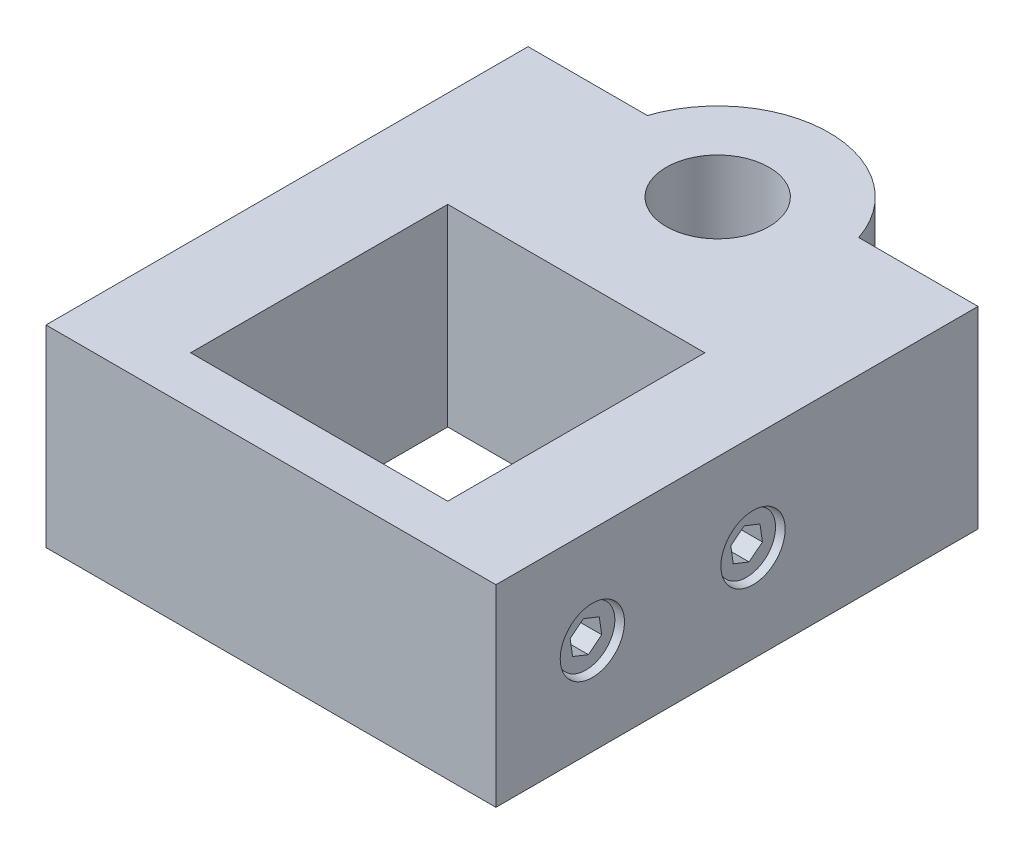
SolidWorks part; units mm, degrees
ref_plane "Front Plane" through (0, 0, 0) normal (0, 0, 1) x (1, 0, 0)
ref_plane "Top Plane" through (0, 0, 0) normal (0, 1, 0) x (1, 0, 0)
ref_plane "Right Plane" through (0, 0, 0) normal (1, 0, 0) x (0, 0, -1)
other "Configuration Table"
sketch "Sketch1" plane through (0, 0, 0) normal (0, 1, 0) x (1, 0, 0)
  line L1 (-35, 27.5) -> (35, 27.5)
  line L2 (-35, 27.5) -> (-35, -27.5)
  line L3 (-35, -27.5) -> (35, -27.5)
  line L4 (35, 27.5) -> (35, -27.5)
  line L5 (-35, 27.5) -> (35, -27.5) construction
  line L6 (-35, -27.5) -> (35, 27.5) construction
  line L7 (-20, 20) -> (20, 20)
  line L8 (-20, 20) -> (-20, -20)
  line L9 (-20, -20) -> (20, -20)
  line L10 (20, 20) -> (20, -20)
  line L11 (-20, 20) -> (20, -20) construction
  line L12 (-20, -20) -> (20, 20) construction
  point P0 (0, 0)
  point P6 (0, 0)
  dimension "D1" = 40
  dimension "D2" = 55
  dimension "D3" = 40
  dimension "D4" = 70
extrude "Boss-Extrude1" add sketch "Sketch1" along normal blind 30
sketch "Sketch2" plane through (0, 30, 0) normal (0, 1, 0) x (1, 0, 0)
  line L0 (-35, 27.5) -> (35, 27.5)
  line L1 (-35, 27.5) -> (-35, 47.5)
  line L2 (35, 27.5) -> (35, 47.5)
  line L3 (-35, 47.5) -> (35, 47.5)
  dimension "D1" = 20
extrude "Boss-Extrude2" add sketch "Sketch2" against normal blind 30
sketch "Sketch3" plane through (0, 0, 0) normal (0, -1, 0) x (1, 0, 0)
  line L0 (20, -20) -> (-20, -20) construction
  circle A0 centre (0, -42) radius 8
  dimension "D1" = 16
  dimension "D2" = 22
extrude "Cut-Extrude1" cut sketch "Sketch3" against normal blind 30
sketch "Sketch4" plane through (0, 0, 0) normal (0, -1, 0) x (1, 0, 0)
  circle A0 centre (0, -42) radius 8
  circle A1 centre (0, -42) radius 17.3384
extrude "Boss-Extrude3" add sketch "Sketch4" against normal blind 30
sketch "Sketch5" plane through (-35, 0, 0) normal (-1, 0, 0) x (0, 0, 1)
  line L0 (27.5, 15) -> (-47.5, 15) construction
  line L1 (27.5, 30) -> (27.5, 0) construction
  line L2 (-47.5, 0) -> (-47.5, 30) construction
  circle A0 centre (12.5, 15) radius 5
  circle A1 centre (-12.5, 15) radius 5
  dimension "D3" = 10
  dimension "D4" = 10
  dimension "D1" = 15
  dimension "D2" = 25
extrude "Cut-Extrude2" cut sketch "Sketch5" against normal blind 6
sketch "Sketch6" plane through (-29, 0, 0) normal (-1, 0, 0) x (0, 0, 1)
  line L1 (-10.4228, 13.3558) -> (-10.0374, 15.9768)
  line L2 (-10.0374, 15.9768) -> (-12.1147, 17.6211)
  line L3 (-12.1147, 17.6211) -> (-14.5772, 16.6442)
  line L4 (-14.5772, 16.6442) -> (-14.9626, 14.0232)
  line L5 (-14.9626, 14.0232) -> (-12.8853, 12.3789)
  line L6 (-12.8853, 12.3789) -> (-10.4228, 13.3558)
  line L7 (14.5697, 13.3558) -> (14.9588, 15.9703)
  line L8 (14.9588, 15.9703) -> (12.8891, 17.6145)
  line L9 (12.8891, 17.6145) -> (10.4303, 16.6442)
  line L10 (10.4303, 16.6442) -> (10.0412, 14.0297)
  line L11 (10.0412, 14.0297) -> (12.1109, 12.3855)
  line L12 (12.1109, 12.3855) -> (14.5697, 13.3558)
  circle A0 centre (-12.5, 15) radius 4.5
  circle A1 centre (12.5, 15) radius 4.5
  circle A2 centre (-12.5, 15) radius 2.2943 construction
  circle A3 centre (12.5, 15) radius 2.2892 construction
  dimension "D1" = 9
  dimension "D2" = 9
extrude "Boss-Extrude4" add sketch "Sketch6" along normal blind 5
mirror "Mirror1" about plane through (0, 0, 0) normal (1, 0, 0) of "Cut-Extrude2", "Boss-Extrude4"
